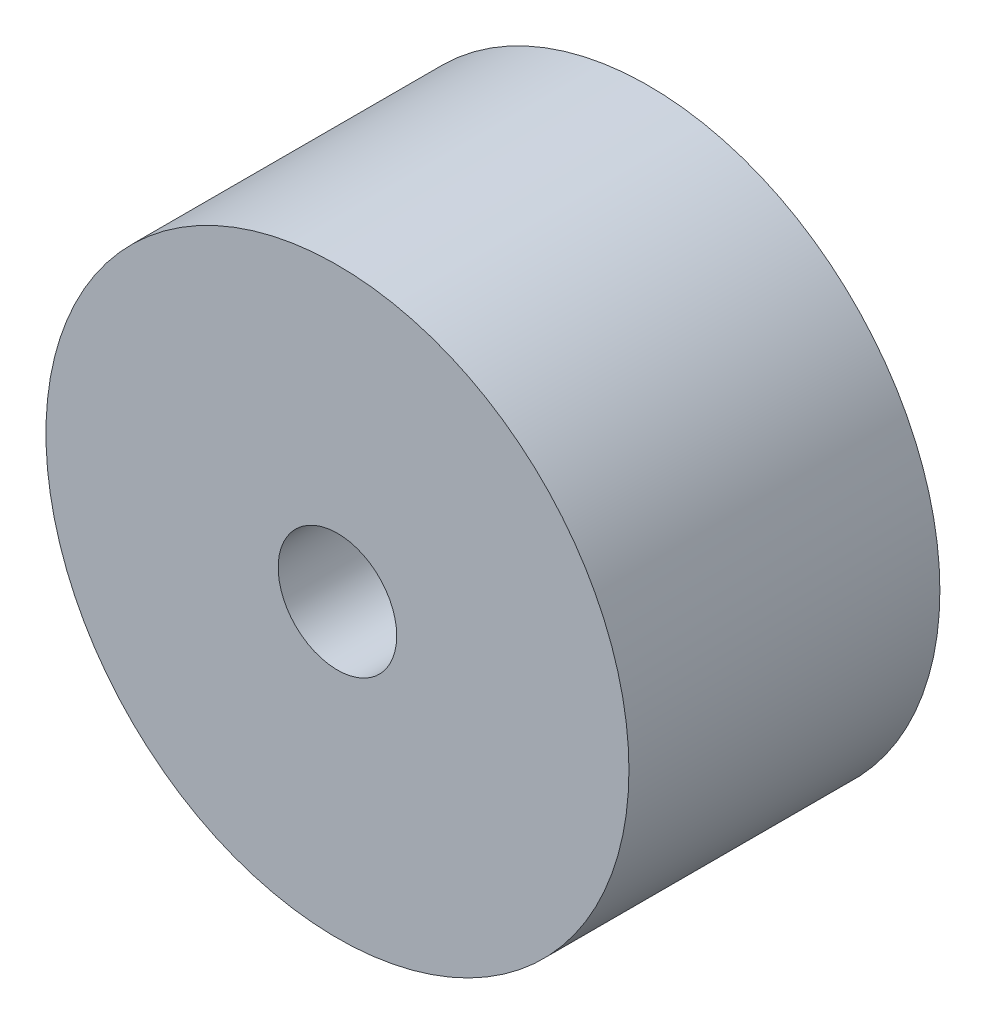
SolidWorks part; units mm, degrees
ref_plane "前视基准面" through (0, 0, 0) normal (0, 0, 1) x (1, 0, 0)
ref_plane "上视基准面" through (0, 0, 0) normal (0, 1, 0) x (1, 0, 0)
ref_plane "右视基准面" through (0, 0, 0) normal (1, 0, 0) x (0, 0, -1)
other "Configuration Table"
sketch "草图1" plane through (0, 0, 0) normal (0, 0, 1) x (1, 0, 0)
  circle A0 centre (0, 0) radius 30
  circle A1 centre (0, 0) radius 6.1
  point P0 (0, 0)
  dimension "D1" = 12.2
  dimension "D2" = 60
extrude "凸台-拉伸1" add sketch "草图1" against normal mid plane 32
